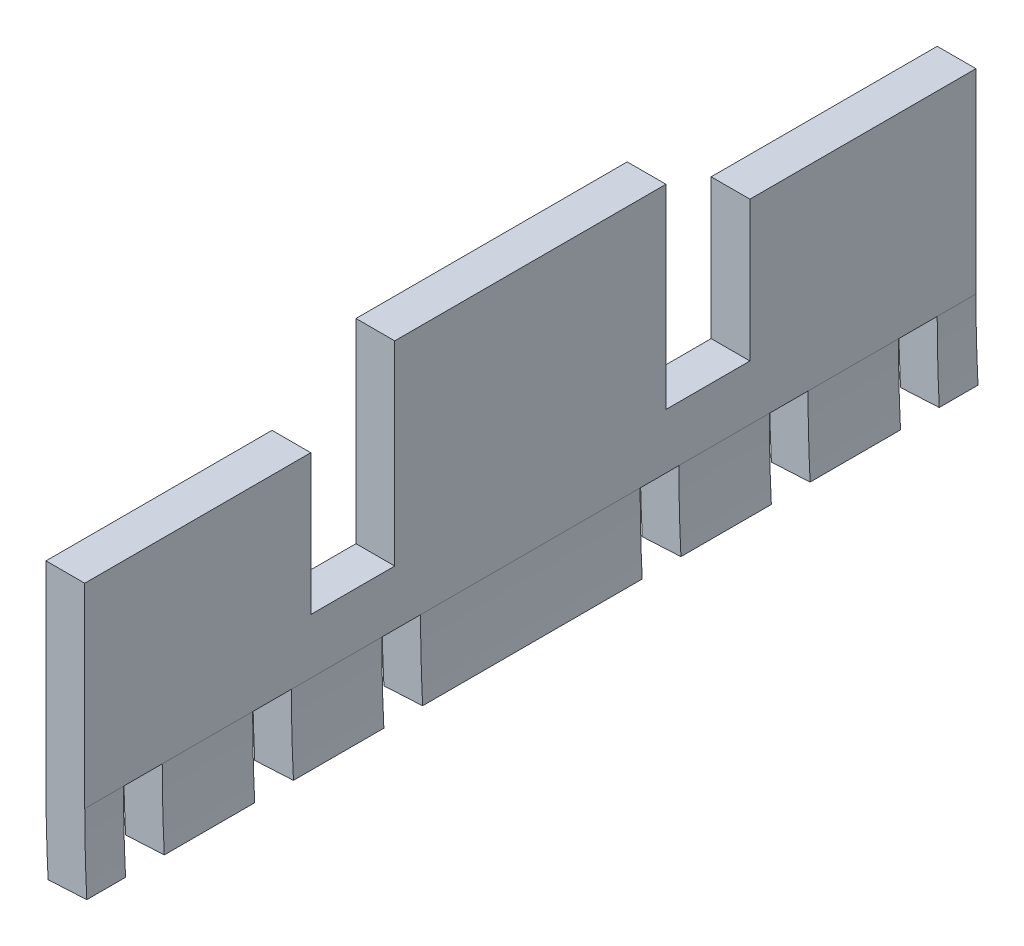
from build123d import *

# Parameters (mm, degrees)
BOSS_EXTRUDE1_DEPTH = 69
SKETCH5_W           = 6
SKETCH5_H           = 28.749782116
CUT_EXTRUDE5_DEPTH  = 250.384613791
CUT_EXTRUDE1_DEPTH  = 80.350082519


with BuildPart() as part:
    # Sketch1 → Boss-Extrude1 (new, symmetric)
    with BuildSketch(Plane.XY):
        with BuildLine():
            Line((-236.175884969, -12.377453651), (-230.184107761, -12.063437914))
            ThreePointArc((-230.184107761, -12.063437914), (-230.421013407, -6.033786585), (-230.5, 0))
            Line((-230.5, 0), (-230.5, 38.722546349))
            Line((-230.5, 38.722546349), (-236.5, 38.722546349))
            Line((-236.5, 38.722546349), (-236.5, 0))
            ThreePointArc((-236.5, 0), (-236.418957357, -6.190848275), (-236.175884969, -12.377453651))
        make_face()
    extrude(amount=BOSS_EXTRUDE1_DEPTH, both=True)

    # Sketch5 → Cut-Extrude5 (cut, through all)
    with BuildSketch(Plane(origin=(0, 0, 0), x_dir=(0, 0, -1), z_dir=(1, 0, 0))):
        with Locations((-60, -14.374891058)):
            Rectangle(SKETCH5_W, SKETCH5_H)
        with Locations((-40, -14.374891058)):
            Rectangle(SKETCH5_W, SKETCH5_H)
        with Locations((-20, -14.374891058)):
            Rectangle(SKETCH5_W, SKETCH5_H)
        with Locations((20, -14.374891058)):
            Rectangle(SKETCH5_W, SKETCH5_H)
        with Locations((40, -14.374891058)):
            Rectangle(SKETCH5_W, SKETCH5_H)
        with Locations((60, -14.374891058)):
            Rectangle(SKETCH5_W, SKETCH5_H)
    extrude(amount=-CUT_EXTRUDE5_DEPTH, mode=Mode.SUBTRACT)

    # Sketch3 → Cut-Extrude1 (cut, through all)
    with BuildSketch(Plane(origin=(-230.5, 0, 0), x_dir=(0, 0, -1), z_dir=(1, 0, 0))):
        Polygon((-69, 30.222546349), (-34, 30.222546349), (-34, 8.522546349), (-21, 8.522546349), (-21, 38.722546349), (-69, 38.722546349), align=None)
        Polygon((21, 8.522546349), (21, 38.722546349), (69, 38.722546349), (69, 30.222546349), (34, 30.222546349), (34, 8.522546349), align=None)
    extrude(amount=-CUT_EXTRUDE1_DEPTH, mode=Mode.SUBTRACT)


solid = part.part
